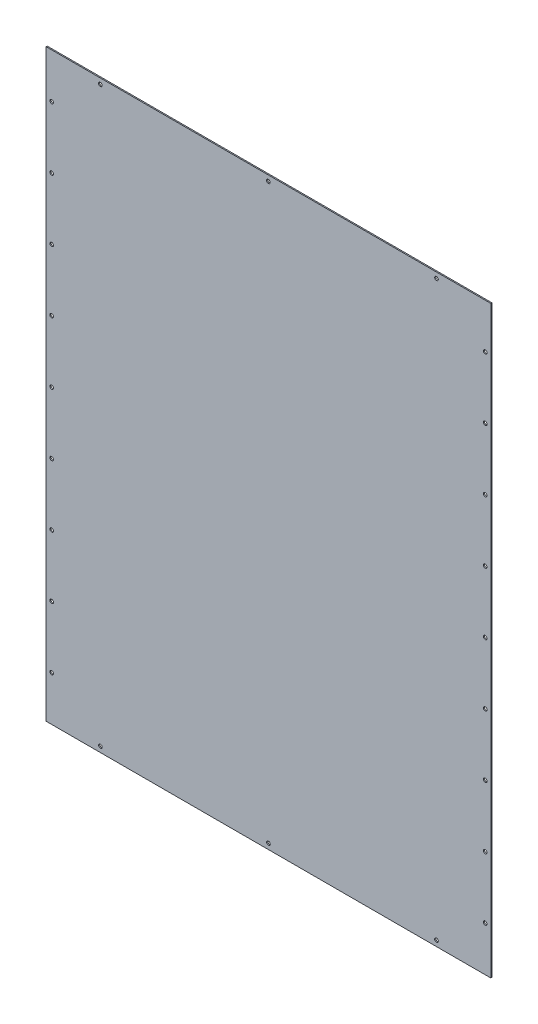
SolidWorks part; units mm, degrees
material "304"
ref_plane "前视基准面" through (0, 0, 0) normal (0, 0, 1) x (1, 0, 0)
ref_plane "上视基准面" through (0, 0, 0) normal (0, 1, 0) x (1, 0, 0)
ref_plane "右视基准面" through (0, 0, 0) normal (1, 0, 0) x (0, 0, -1)
sketch "草图1" plane through (0, 0, 0) normal (0, 0, 1) x (1, 0, 0)
  line L0 (0, 0) -> (451.2544, 0) construction
  line L1 (-397, 521.5) -> (397, 521.5)
  line L2 (-397, 521.5) -> (-397, -521.5)
  line L3 (-397, -521.5) -> (397, -521.5)
  line L4 (397, 521.5) -> (397, -521.5)
  line L5 (-397, 521.5) -> (397, -521.5) construction
  line L6 (-397, -521.5) -> (397, 521.5) construction
  line L7 (0, 0) -> (0, 412.8629) construction
  circle A0 centre (-387, 0) radius 3.25
  circle A1 centre (-387, -110.375) radius 3.25
  circle A2 centre (-387, -220.75) radius 3.25
  circle A3 centre (-387, -331.125) radius 3.25
  circle A4 centre (-387, -441.5) radius 3.25
  circle A34 centre (0, -511.5) radius 3.25
  circle A35 centre (0, 511.5) radius 3.25
  circle A36 centre (-387, 441.5) radius 3.25
  circle A37 centre (-387, 331.125) radius 3.25
  circle A38 centre (-387, 220.75) radius 3.25
  circle A39 centre (-387, 110.375) radius 3.25
  circle A40 centre (387, 110.375) radius 3.25
  circle A41 centre (387, 220.75) radius 3.25
  circle A42 centre (387, 331.125) radius 3.25
  circle A43 centre (387, 441.5) radius 3.25
  circle A44 centre (387, -441.5) radius 3.25
  circle A45 centre (387, -331.125) radius 3.25
  circle A46 centre (387, -220.75) radius 3.25
  circle A47 centre (387, -110.375) radius 3.25
  circle A48 centre (387, 0) radius 3.25
  circle A49 centre (-300, 511.5) radius 3.25
  circle A50 centre (300, 511.5) radius 3.25
  circle A51 centre (300, -511.5) radius 3.25
  circle A52 centre (-300, -511.5) radius 3.25
  point P0 (0, 0)
  dimension "D3" = 6.5
  dimension "D8" = 600
  dimension "D1" = 794
  dimension "D2" = 1043
  dimension "D4" = 10
  dimension "D6" = 10
  dimension "D7" = 80
  dimension "D5" = 5
extrude "凸台-拉伸1" add sketch "草图1" along normal blind 2
